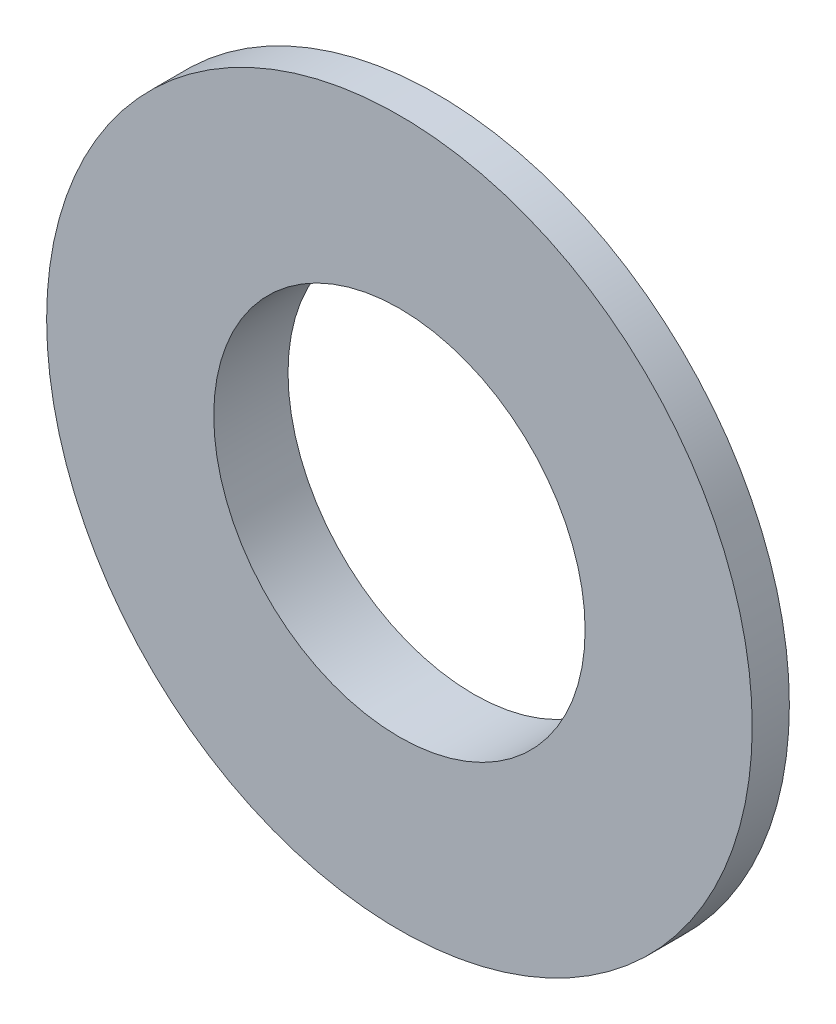
from build123d import *


with BuildPart() as part:
    # Sketch1 → Revolve1 (revolve)
    with BuildSketch(Plane(origin=(0, 234.743963655, 0), x_dir=(1, 0, 0), z_dir=(0, 1, 0))):
        Polygon((546.230642584, 388.998443067), (568.730642584, 388.998443067), (568.730642584, 393.998443067), (554.230642584, 398.998443067), (546.230642584, 398.998443067), align=None)
    revolve(axis=Axis((521.230642584, 234.743963655, -398.998443067), (0, 0, 1)))


solid = part.part
